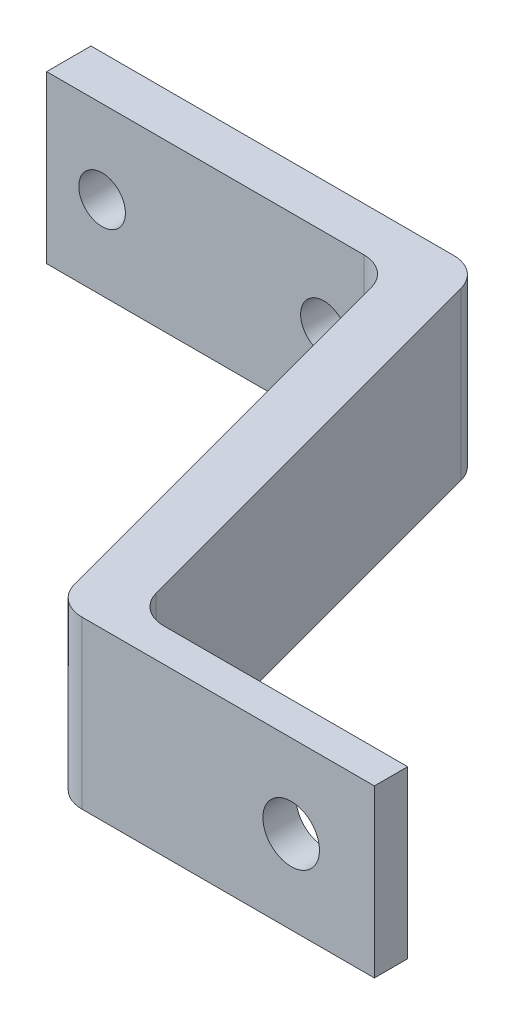
SolidWorks part; units mm, degrees
material "6061 合金"
ref_plane "前视基准面" through (0, 0, 0) normal (0, 0, 1) x (1, 0, 0)
ref_plane "上视基准面" through (0, 0, 0) normal (0, 1, 0) x (1, 0, 0)
ref_plane "右视基准面" through (0, 0, 0) normal (1, 0, 0) x (0, 0, -1)
other "Configuration Table"
sketch "草图1" plane through (0, 0, 0) normal (0, 1, 0) x (1, 0, 0)
  line L0 (0, 0) -> (0, -4)
  line L1 (0, -4) -> (30.8954, -4)
  line L2 (30.8954, -4) -> (41.8813, -45)
  line L3 (41.8813, -45) -> (70.55, -45)
  line L4 (70.55, -45) -> (70.55, -42)
  line L5 (70.55, -42) -> (46.2539, -42)
  line L6 (46.2539, -42) -> (35, 0)
  line L7 (35, 0) -> (0, 0)
  dimension "D1" = 4
  dimension "D2" = 3
  dimension "D3" = 5
  dimension "D4" = 105
  dimension "D5" = 42
  dimension "D6" = 35
  dimension "D7" = 35.55
extrude "凸台-拉伸1" add sketch "草图1" along normal blind 15
sketch "草图2" plane through (0, 0, 42) normal (0, 0, -1) x (-1, 0, 0)
  line L0 (-70.55, 15) -> (-70.55, 0) construction
  line L1 (-70.55, 0) -> (-46.2539, 0) construction
  line L2 (0, 15) -> (0, 0) construction
  circle A0 centre (-63.05, 7.5) radius 2.55
  circle A1 centre (-25, 7.5) radius 2.1
  circle A2 centre (-5, 7.5) radius 2.1
  point P6 (0, 0)
  point P7 (-2.2457, 7.0398)
  point P10 (-17.4134, 7.1598)
  point P13 (-4.6634, 7.5)
  dimension "D1" = 5.1
  dimension "D3" = 4.2
  dimension "D2" = 20
  dimension "D4" = 7.5
  dimension "D5" = 7.5
  dimension "D6" = 5
extrude "切除-拉伸1" cut sketch "草图2" against normal through all both and the other way through all
fillet "圆角1" radius 3 4 edges at (41.8813, 7.5, 45) (46.2539, 7.5, 42) (35, 7.5, 0) (30.8954, 7.5, 4)
